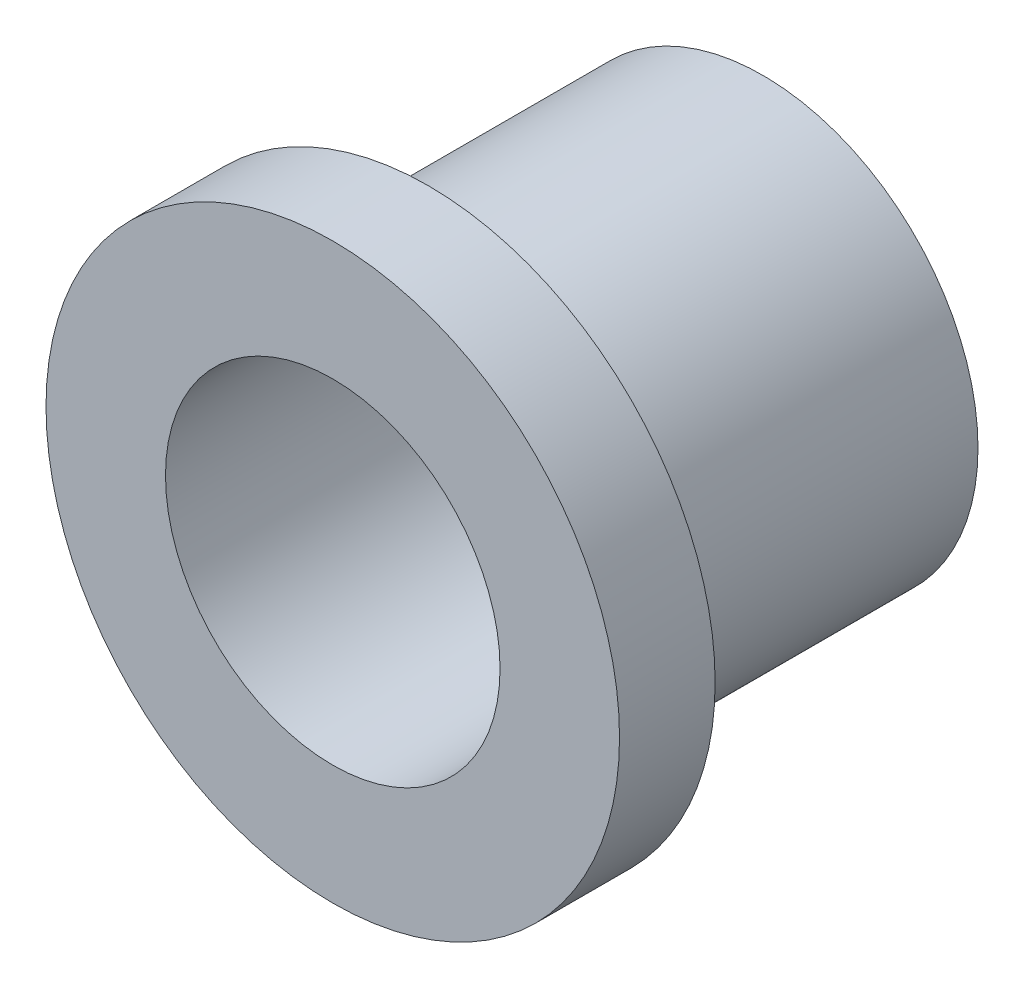
SolidWorks part; units mm, degrees
ref_plane "前视基准面" through (0, 0, 0) normal (0, 0, 1) x (1, 0, 0)
ref_plane "上视基准面" through (0, 0, 0) normal (0, 1, 0) x (1, 0, 0)
ref_plane "右视基准面" through (0, 0, 0) normal (1, 0, 0) x (0, 0, -1)
other "Configuration Table"
sketch "草图1" plane through (0, 0, 0) normal (0, 0, 1) x (1, 0, 0)
  circle A0 centre (0, 0) radius 6
  circle A1 centre (0, 0) radius 3.5
  point P0 (0, 0)
  dimension "D1" = 7
  dimension "D2" = 12
extrude "凸台-拉伸1" add sketch "草图1" against normal mid plane 2
sketch "草图2" plane through (0, 0, 0) normal (0, 0, 1) x (1, 0, 0)
  circle A0 centre (0, 0) radius 4.5
  circle A1 centre (0, 0) radius 3.5
  point P0 (0, 0)
  dimension "D1" = 7
  dimension "D2" = 9
extrude "凸台-拉伸2" add sketch "草图2" against normal blind 8
